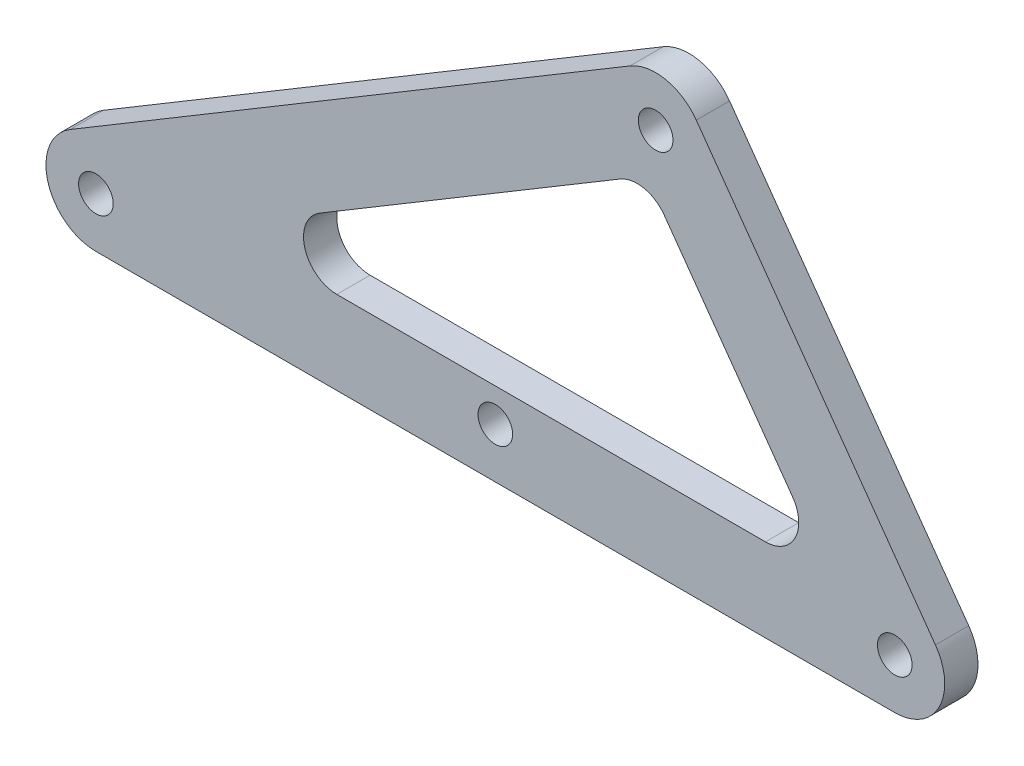
SolidWorks part; units mm, degrees
ref_plane "Front Plane" through (0, 0, 0) normal (0, 0, 1) x (1, 0, 0)
ref_plane "Top Plane" through (0, 0, 0) normal (0, 1, 0) x (1, 0, 0)
ref_plane "Right Plane" through (0, 0, 0) normal (1, 0, 0) x (0, 0, -1)
other "Configuration Table"
sketch "Sketch1" plane through (0, 0, 0) normal (0, 0, 1) x (1, 0, 0)
  line L0 (0, 0) -> (-84.0796, -50.3076) construction
  line L1 (-84.0796, -50.3076) -> (-24.0796, -50.3076) construction
  line L2 (-24.0796, -50.3076) -> (35.9204, -50.3076) construction
  line L3 (35.9204, -50.3076) -> (0, 0) construction
  line L4 (42.0242, -45.9494) -> (6.1038, 4.3582)
  line L5 (-3.8508, 6.4359) -> (-87.9305, -43.8717)
  line L6 (-84.0796, -57.8076) -> (-24.0796, -57.8076)
  line L7 (-24.0796, -57.8076) -> (35.9204, -57.8076)
  line L8 (-5.3466, -9.0257) -> (-50.4574, -36.017)
  line L9 (2.0845, 9.9873) -> (-111.2217, -57.8076) construction
  line L10 (-111.2217, -57.8076) -> (-24.0796, -57.8076) construction
  line L11 (50.4911, -57.8076) -> (2.0845, 9.9873) construction
  line L12 (-24.0796, -57.8076) -> (50.4911, -57.8076) construction
  line L13 (-47.8902, -45.3076) -> (-24.0796, -45.3076)
  line L14 (-24.0796, -45.3076) -> (16.4928, -45.3076)
  line L15 (20.562, -37.4021) -> (1.2898, -10.4109)
  line L16 (-24.0796, -45.3076) -> (26.2066, -45.3076) construction
  line L17 (26.2066, -45.3076) -> (-1.3897, -6.6582) construction
  line L18 (-65.9849, -45.3076) -> (-24.0796, -45.3076) construction
  line L19 (-1.3897, -6.6582) -> (-65.9849, -45.3076) construction
  circle A0 centre (-84.0796, -50.3076) radius 2.6
  circle A1 centre (-24.0796, -50.3076) radius 2.6
  circle A2 centre (35.9204, -50.3076) radius 2.6
  arc A4 (6.1038, 4.3582) -> (-3.8508, 6.4359) centre (0, 0) ccw
  arc A5 (-87.9305, -43.8717) -> (-84.0796, -57.8076) centre (-84.0796, -50.3076) ccw
  arc A7 (35.9204, -57.8076) -> (42.0242, -45.9494) centre (35.9204, -50.3076) ccw
  circle A9 centre (0, 0) radius 2.6
  arc A11 (16.4928, -45.3076) -> (20.562, -37.4021) centre (16.4928, -40.3076) ccw
  arc A12 (-47.8902, -45.3076) -> (-50.4574, -36.017) centre (-47.8902, -40.3076) cw
  arc A13 (1.2898, -10.4109) -> (-5.3466, -9.0257) centre (-2.7794, -13.3163) ccw
  dimension "D5" = 5.2
  dimension "D6" = 15
  dimension "D9" = 5
  dimension "D1" = 35.9204
  dimension "D2" = 50.3076
  dimension "D3" = 84.0796
  dimension "D4" = 24.0796
  dimension "D7" = 7.5
  dimension "D8" = 5
extrude "Boss-Extrude1" add sketch "Sketch1" along normal blind 5
